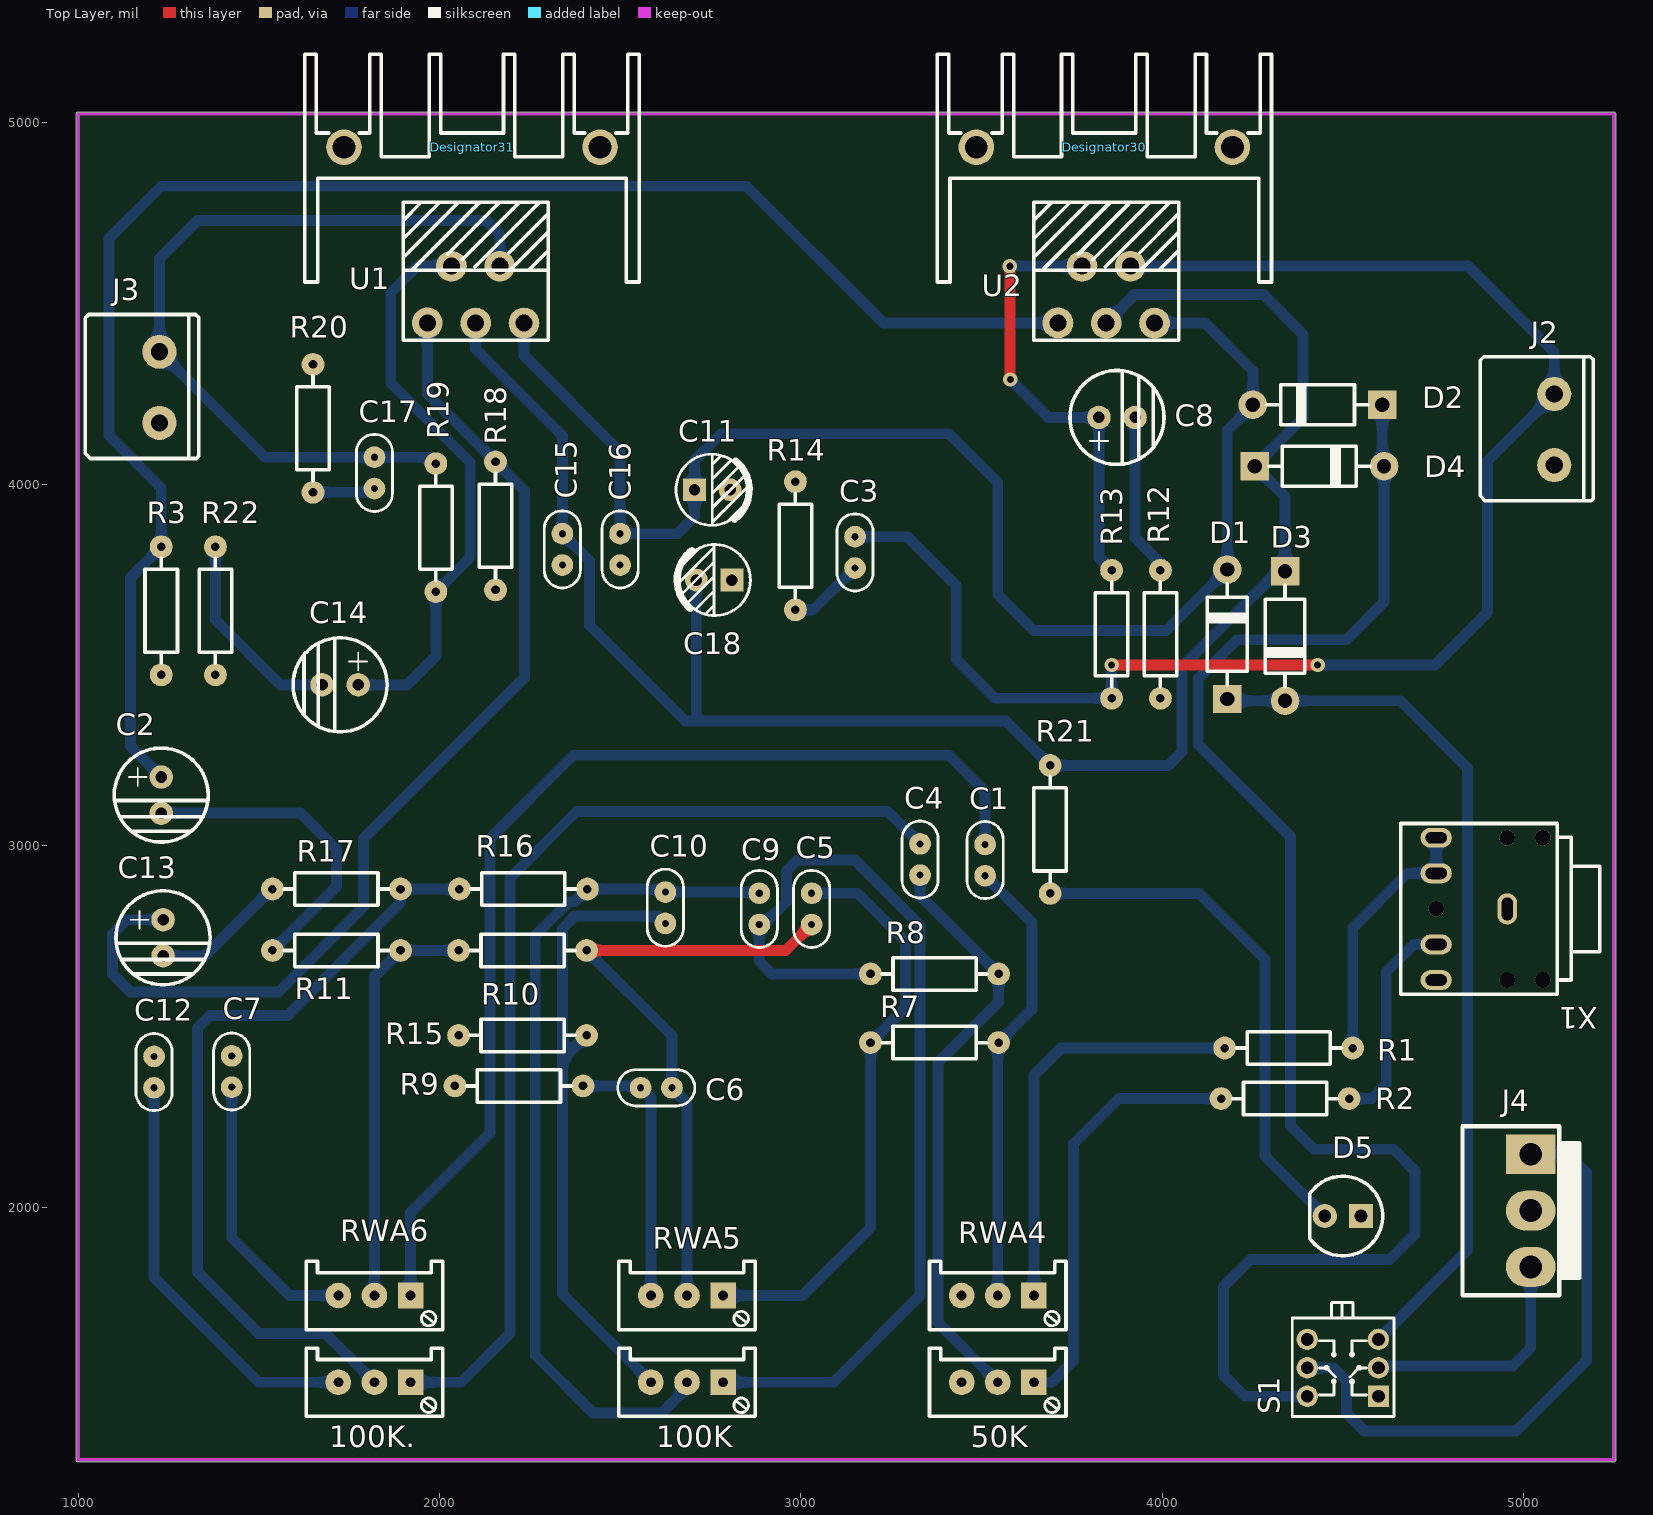
[diagram p0: Top Layer view]
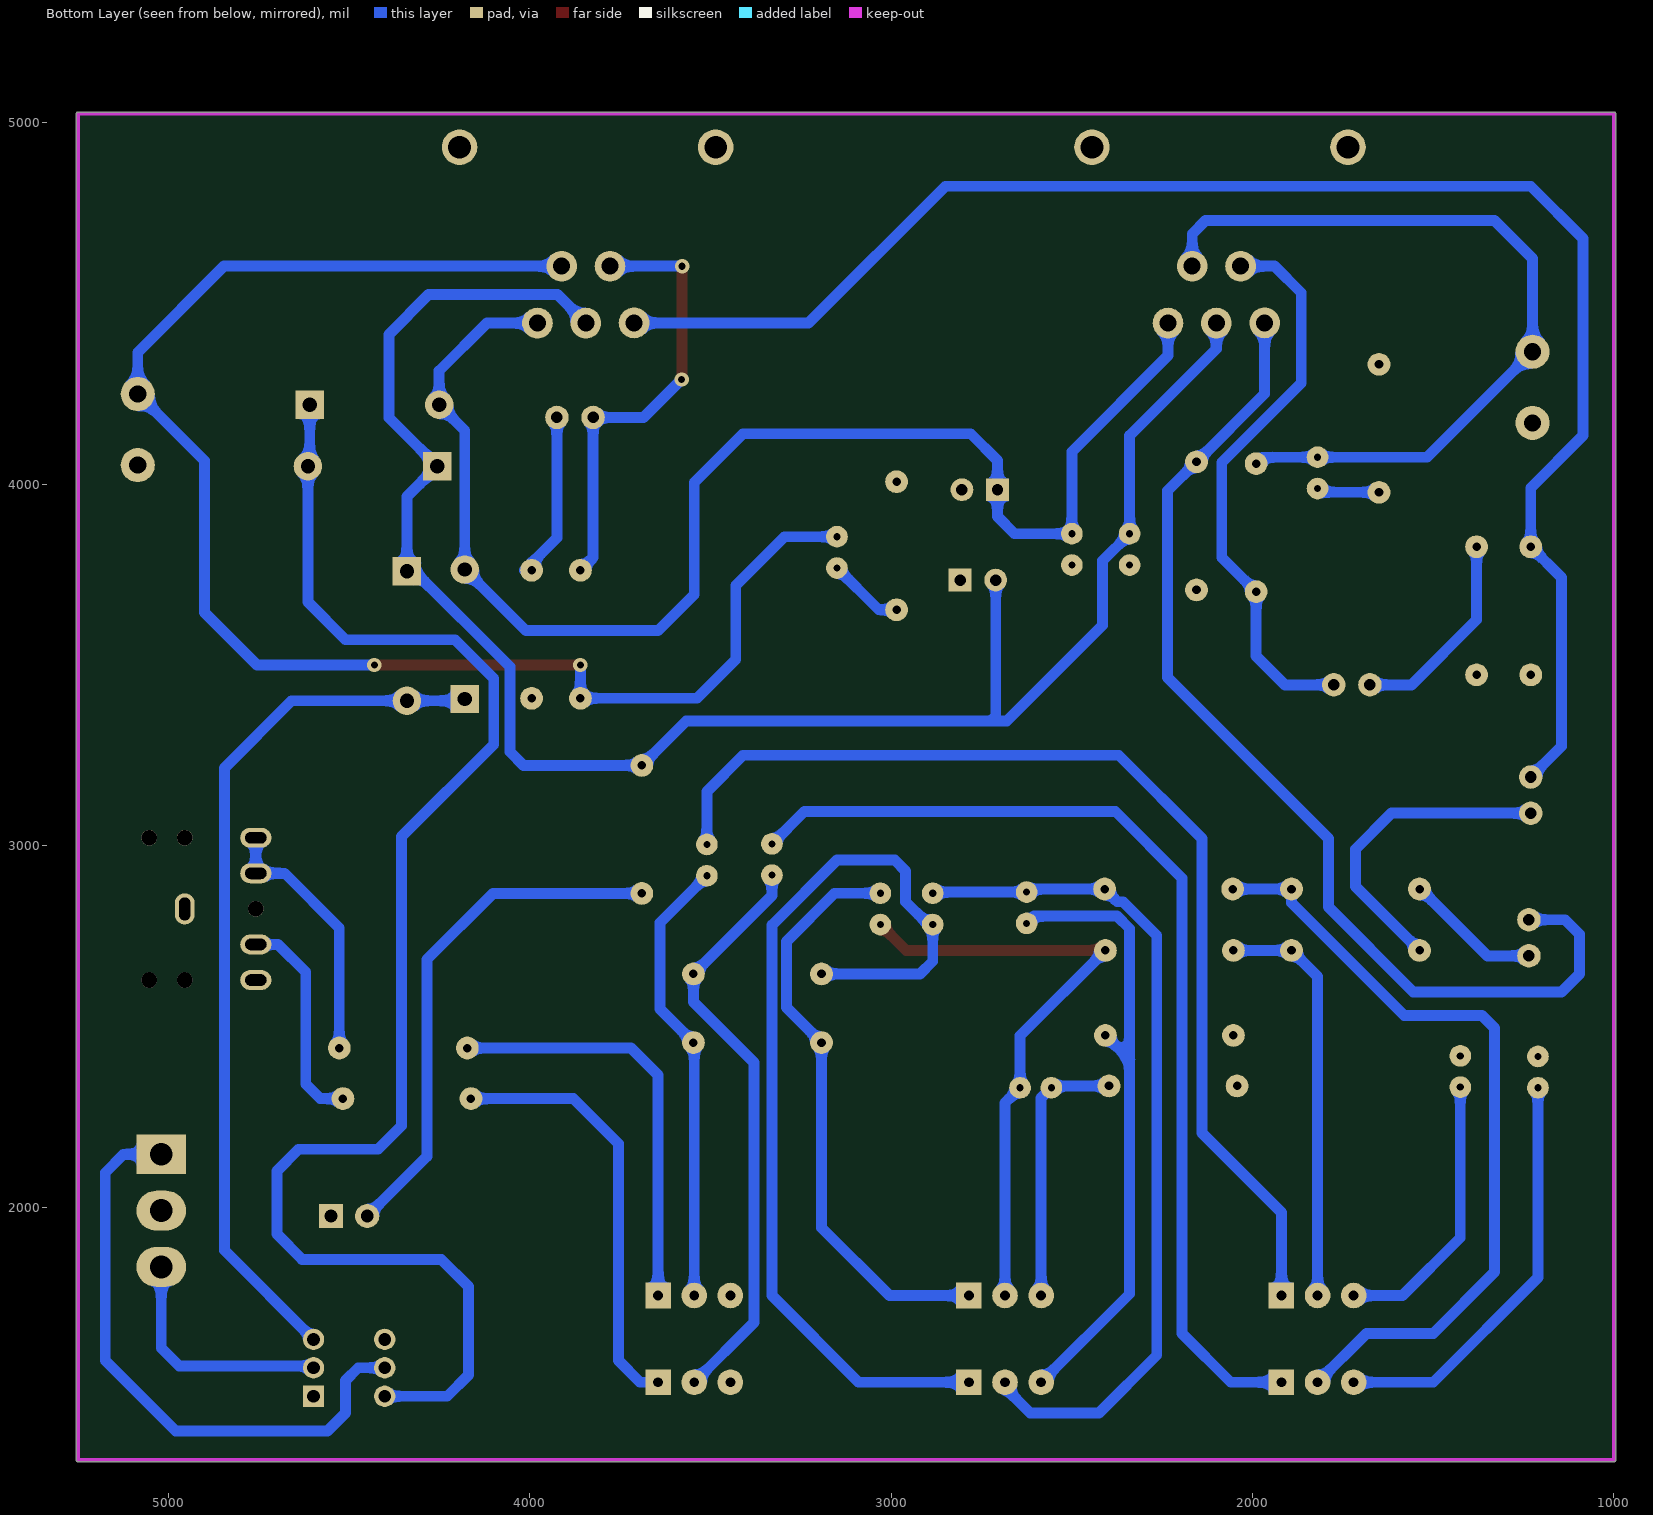
[diagram p1: Bottom Layer view, seen from below]
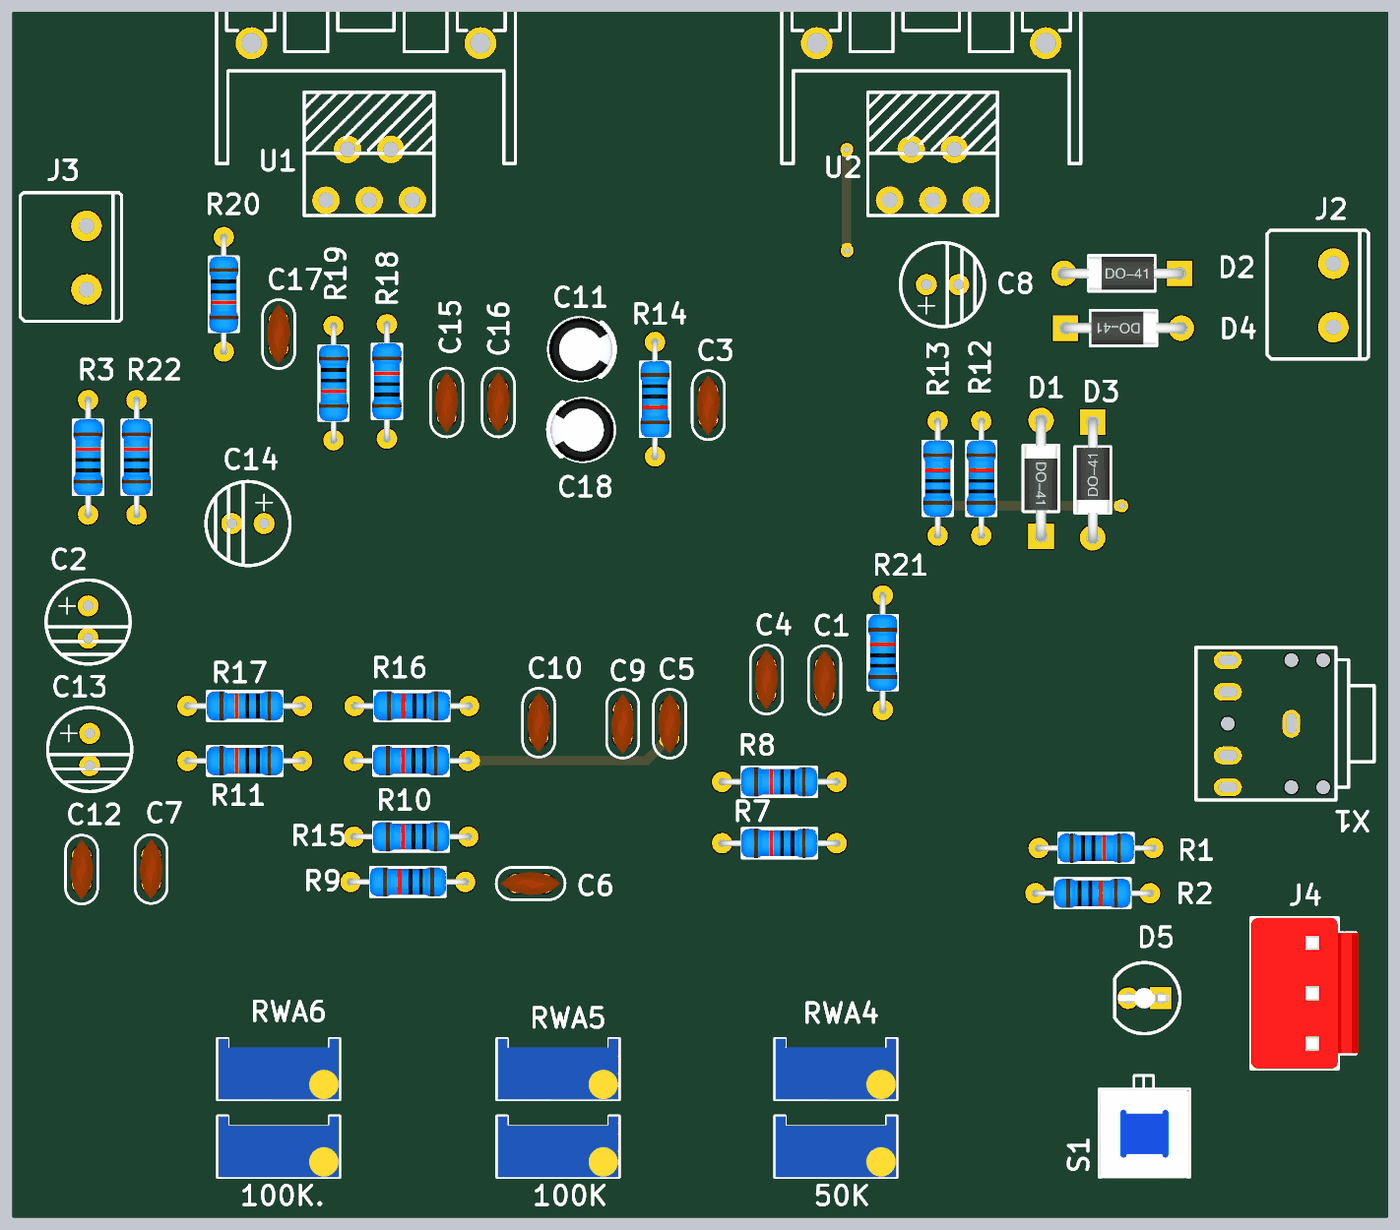
[diagram p2: 3D render of the assembled board from above, using the file's embedded part models]
# Altium PCB MISC82779.PcbDoc
Units mil, origin at the board's own origin, x right, y up, seen from the top; angles counter-clockwise.
Board outline 4260.03 x 3735.03 mil, 2 copper layers (Top Layer, Bottom Layer); 57 components, 38 nets, 139 pads, 4 vias.

## Layer stack, top to bottom (the 12.6 mil dielectric is the usual default, probably not edited)
Top Solder: solder mask 0.4, Solder Resist, Dk 3.5
Top Layer: signal copper 1.4
Dielectric 1: dielectric 12.6, FR-4, Dk 4.8
Bottom Layer: signal copper 1.4
Bottom Solder: solder mask 0.4, Solder Resist, Dk 3.5

## Board outline
1000,1294.98 cw(c1000,1300) 994.99,1300 994.99,5025 cw(c1000,5025) 1000,5030.02 5250,5030.02 cw(c5250,5025) 5255.02,5025 5255.02,1300 cw(c5250,1300) 5250,1294.98

## Design rules (kind name [scope] priority, off if disabled: settings)
Clearance [All] p1: gap=10
HoleSize [All] p1: absolutevalues=TRUE maxlimit=9999 minlimit=1 maxpercent=80.000 minpercent=20.000
MinimumSolderMaskSliver [All] p1: minsoldermaskwidth=9
PolygonConnect [All] p1: connectstyle=Relief reliefconductorwidth=10 reliefentries=4 polygonreliefangle="90 Angle" airgapwidth=10
RoutingVias [All] p1: holewidth=28 width=50 viastyle="Through Hole" minholewidth=28 minwidth=50 maxholewidth=28 maxwidth=50
SilkToSilkClearance [All] p1: silktosilkclearance=0
SilkToSolderMaskClearance [IsPad] p1: minsilkscreentomaskgap=9 clearancetoexposedcopper=TRUE
SolderMaskExpansion [All] p1: expansion=4
Width [All] p1: maxlimit=30 minlimit=10 preferedwidth=10
26 further rules are at their usual default settings.

## Components (designator, comment, footprint, x,y, rotation, side; value= is the part's Value field where it differs from the comment)
50K "10K" 3296W 3545,1515 r180 top
100K "10K" 3296W 2685,1515 r180 top
100K. "10K" 3296W 1820,1515 r180 top
C1 "222" "CC 2.2*5" 3510,2960 r90 top
C2 "10UF" EC100 1230,3090 r0 top
C3 "224" "CC 2.2*5" 3150,3811.69 r90 top
C4 "222" "CC 2.2*5" 3330,2961.69 r90 top
C5 "223" "CC 2.2*5" 3030,2825 r90 top
C6 "224" "CC 2.2*5" 2600,2330 r0 top
C7 "223" "CC 2.2*5" 1425,2375 r270 top
C8 "10UF" EC100 3925,4185 r90 top
C9 "223" "CC 2.2*5" 2885,2825 r270 top
C10 "224" "CC 2.2*5" 2625,2828.31 r90 top
C11 "2200UF" "CAP 2.5*5*11 - BK" 2755,3985 r0 top
C12 "223" "CC 2.2*5" 1210,2373.31 r270 top
C13 "10UF" EC100 1235,2695 r0 top
C14 "10UF" EC100 1675,3445 r270 top
C15 "104" "CC 2.2*5" 2340,3820 r90 top
C16 "104" "CC 2.2*5" 2500,3820 r90 top
C17 "224" "CC 2.2*5" 1820,4031.69 r90 top
C18 "2200UF" "CAP 2.5*5*11 - BK" 2760,3735 r180 top
D1 "1N4007" DO-41 4180,3585 r90 top
D2 "1N4007" DO-41 4430,4220 r180 top
D3 "1N4007" DO-41 4340,3580 r270 top
D4 "1N4007" DO-41 4435,4050 r0 top
D5 "LED" "LED 5MM-W" 4500,1975 r180 top
Designator30 "Comment" TH-2P_L23.5-W16.8 3840,4875 r0 top
Designator31 "Comment" TH-2P_L23.5-W16.8 2090,4875 r0 top
J2 "socket" DZ 5085,4053.15 r90 top
J3 "socket" DZ 1225,4170 r90 top
J4 "AC+/-12V" VH3.96-3A 5020,2145.91 r270 top
R1 "1K" "RS 1/4W" 4350,2440 r0 top
R2 "1K" "RS 1/4W" 4340,2300 r0 top
R3 "22K" "RS 1/4W" 1230,3650 r90 top
R7 "10K" "RS 1/4W" 3370,2455 r180 top
R8 "10K" "RS 1/4W" 3370,2645 r180 top
R9 "1.5K" "RS 1/4W" 2220,2335 r180 top
R10 "5.6K" "RS 1/4W" 2230,2710 r180 top
R11 "2.2K" "RS 1/4W" 1715,2710 r180 top
R12 "330" "RS 1/4W" 3995,3585 r90 top
R13 "47K" "RS 1/4W" 3860,3585 r90 top
R14 "10" "RS 1/4W" 2985,3830 r270 top
R15 "1.5K" "RS 1/4W" 2230,2475 r180 top
R16 "5.6K" "RS 1/4W" 2232.17,2880 r180 top
R17 "2.2K" "RS 1/4W" 1715,2880 r180 top
R18 "22K" "RS 1/4W" 2155,3885 r90 top
R19 "47K" "RS 1/4W" 1990,3880 r270 top
R20 "10" "RS 1/4W" 1650,4155 r270 top
R21 "10K" "RS 1/4W" 3690,3045 r90 top
R22 "330" "RS 1/4W" 1380,3650 r90 top
RWA4 "10K" 3296W 3545,1755 r180 top
RWA5 "10K" 3296W 2685,1755 r180 top
RWA6 "10K" 3296W 1820,1755 r180 top
S1 "KET 7X7" "KFT DIP-7X7" 4500,1555 r90 top
U1 "TDA2030" TDA2030 2100,4590 r0 top
U2 "TDA2030" TDA2030 3845,4590 r0 top
X1 "STEREO" 3F07 4935.31,2825 r180 top

## Footprints (in the part's own frame and the unit in brackets; to place one, negate y for a bottom-side part, rotate by r counter-clockwise, add the part's x,y. Pads: shape width x height; smd on the part's side, far side on the other; paste and mask are expansions set on the pad)
3F07 [mm]
  oval 1.4x2.2 hole 0.8 slot 1.6 at 90 deg paste+0 mask+0.051: 1(-0.5,0)
  oval 2.2x1.4 hole 0.8 slot 1.5 at 0 deg paste+0 mask+0.051: 2(4.5,5) 3(4.5,2.5) 4(4.5,-2.5) 5(4.5,-5)
  round 1.1 hole 1.1 unplated paste+0: ""(-3,5) ""(-3,-5) ""(-0.5,5) ""(-0.5,-5) ""(4.5,0)
  silkscreen extent -7,-6 7,6
3296W [mm] "Precise Multi-Winding Adjustable Resistor"
  rect 1.8x1.8 hole 0.7: 1(-2.54,0)
  round 1.8 hole 0.7: 2(0,0) 3(2.54,0)
  silkscreen extent -4.8,-2.4 4.8,2.4, body extent -4.75,-2.4 4.75,2.4, height 11.52
"CAP 2.5*5*11 - BK" [mm] "脚距2.5mm直径5mm高度11mm"
  rect 1.6x1.6 hole 0.8: 1(-1.25,0)
  round 1.6 hole 0.8: 2(1.25,0)
  silkscreen extent -2.55,-2.5 2.6,2.5, body extent -2.5,-2.5 2.51,2.5, height 11.04
"CC 2.2*5" [mil] "脚距2.2mm直径5mm"
  round 60 hole 19.68: 1(-43.31,0) 2(43.31,0)
  silkscreen extent -107,-50 107,50, body extent -94,-36 94,36, height 189
DO-41 [mm] "2.6*9.1mm(直径，脚距）"
  rect 2x2 hole 1: 1(-4.55,0)
  round 2 hole 1: 2(4.55,0)
  silkscreen extent -3.56,-1.4 3.56,1.4, body extent -4.92,-1.29 4.98,1.31, height 2.65
DZ [mm]
  round 2.4 hole 1.2: 1(0,0) 2(5,0)
  silkscreen extent -2.5,-2.75 7.62,5.21
EC100 [mil]
  round 65 hole 32: 1(0,100) 2(0,0)
  silkscreen extent -130,-80 130,180
"KFT DIP-7X7" [mm] "自锁开关，规格：7*7mm"
  rect 1.5x1.5 hole 0.9: 1(-2,-2.5)
  round 1.5 hole 0.9: 2(0,-2.5) 3(2,-2.5) 4(2,2.5) 5(0,2.5) 6(-2,2.5)
  silkscreen extent -3.42,-3.58 4.58,3.56, body extent -3.5,-3.5 3.5,3.5, height 11.2
"LED 5MM-W" [mm] "白色5mm直插LED"
  rect 1.7x1.7 hole 0.9: 1(-1.27,0)
  round 1.7 hole 0.9: 2(1.27,0)
  silkscreen extent -2.8,-2.8 2.33,2.8, body extent -2.85,-2.85 2.45,2.85, height 8.75
"RS 1/4W" [mm]
  round 1.6 hole 0.6: 1(-4.5,0) 2(4.5,0)
  silkscreen extent -3.68,-1.14 3.68,1.14, body extent -4.72,-1.16 4.73,1.16, height 2.32
TDA2030 [mil]
  round 85 hole 47.24 paste+0 mask+2: 1(-133.54,-143.46) 2(-66.93,13.78) 3(0,-143.7) 4(66.93,13.78) 5(133.86,-143.7)
  silkscreen extent -201,-191 201,191
TH-2P_L23.5-W16.8 [mm]
  round 2.5 hole 1.6 paste+0 mask+0.05: 1(-8.999,1.47) 2(9.001,1.47)
  silkscreen extent -11.75,-8 11.75,8
VH3.96-3A [mm]
  rect 2.8x3.5 hole 1.6: 1(0,0)
  oval 2.8x3.5 hole 1.6: 2(3.96,0) 3(7.92,0)
  silkscreen extent -1.98,-4.8 9.9,3.4, body extent -1.98,-4.8 9.9,3.6, height 14.6

## Part data
50K 100K 100K. RWA4 RWA5 RWA6: library part RP, "single-gang potentiometer"
C1 C3 C4 C5 C6 C7 C9 C10 C12 C15 C16 C17: library part CC, "ceramic disc capacitor"
C2 C8 C13 C14: library part ECAP
C11 C18: library part CE, "through-hole electrolytic capacitor"
D1 D2 D3 D4: "rectifier diode"
J2 J3: library part 插座
J4: library part VH3
R1 R2 R3 R7 R8 R9 R10 R11 R12 R13 R14 R15 R16 R17 R18 R19 R20 R21 R22: library part R-S, "color-band resistor"
S1: "7*7 self-locking switch"
X1: library part 3F07

## Via types
v1: diameter 40, hole 20, Top Layer to Bottom Layer, 4 vias

## Nets (pads, with @x,y where several pads share a name; then routed paths per layer and width w, separated by ;. In a path a pad name is that pad's centre, name@x,y a point inside that pad or via, vN(x,y) a via of type N, cw(c..) or ccw(c..) an arc to the next point about the centre after c; other vN are vias at no path point)
+17V: C11.1 C16.2 D1.2 D2.2 U1.5 U2.5 | length 3962.1
  Bottom Layer w30: U1.5 2233.86,4356.14 2500,4090 C16.2 2658.31,3863.31 2705.79,3910.79 C11.1 2705.79,4065.79 2780,4140 3410,4140 3545,4005 3545,3695 3645,3595 4010.87,3595 D1.2 4180,4149.13 D2.2 4250.87,4314.13 4118.7,4446.3 U2.5
-17V: C15.2 C18.2 D3.1 D4.1 R21.2 U1.3 U2.3 | length 5177.8
  Bottom Layer w30: U1.3 2100,4375 2340,4135 C15.2 2415,3788.31 2415,3610 2680,3345 2725,3345 ; C18.2 2710.79,3359.21 2725,3345 ; U2.3 3923.7,4525 4280,4525 4390,4415 4390,4184.13 D4.1 4340,3965.87 D3.1 4319.13,3759.13 4055,3495 4055,3260 4017.17,3222.17 R21.2 3567.17,3345 2725,3345
GND: 50K.3 C7.1 C11.2 C12.1 C15.1 C16.1 C18.1 D5.1 J2.1 J3.1 J4.2 R3.1 R9.2 R12.1 R14.1 R15.2 R18.1 R20.1 R22.1 RWA4.3 X1.1
Net50K_1: 50K.1 R2.1 | length 1194.5
  Bottom Layer w30: 50K.1 3695,1515 3755,1575 3755,2175 3880,2300 R2.1
Net50K_2: 50K.2 C4.1 R8.1 | length 1630.9
  Bottom Layer w30: C4.1 3330,2862.17 R8.1 3547.17,2567.17 3380,2400 3380,1680 50K.2
Net100K._1: 100K..1 C4.2 | length 2839.8
  Bottom Layer w30: 100K..1 2060,1515 2195,1650 2195,2910 2380,3095 3240,3095 C4.2
Net100K._2: 100K..2 R16.2 R17.1 | length 2198
  Bottom Layer w30: 100K..2 1685,1650 1500,1650 1330,1820 1330,2495 1365,2530 1580,2530 1892.17,2842.17 R17.1 R16.2
Net100K._3: 100K..3 C12.2 | length 1155.1
  Bottom Layer w30: C12.2 1210,1805 1500,1515 100K..3
Net100K_1: 100K.1 C9.2 R8.2 | length 2741.5
  Bottom Layer w30: 100K.1 3090,1515 3330,1755 3330,2780 3150,2960 2990,2960 2960,2930 2960,2845 2905,2790 2885,2790 C9.2 2885,2680 2920,2645 R8.2
Net100K_2: 100K.2 C9.1 C10.2 R16.1 | length 2369.9
  Bottom Layer w30: 100K.2 2685,1500 2615,1430 2425,1430 2265,1590 2265,2751.57 2358.43,2845 2374.33,2845 R16.1 2616.61,2880 C10.2 2881.69,2871.61 C9.1
Net100K_3: 100K.3 C10.1 R15.1 | length 1759.3
  Bottom Layer w30: R15.1 2340,2407.83 ; 100K.3 2340,1760 2340,2407.83 ; C10.1 2605,2805 2375,2805 2340,2770 2340,2407.83
NetC1_1: C1.1 R7.1 RWA4.2 | length 1254.9
  Bottom Layer w30: C1.1 3640,2786.69 3640,2547.83 R7.1 3545,2452.83 RWA4.2
NetC1_2: C1.2 RWA6.1 | length 3009.5
  Bottom Layer w30: RWA6.1 1920,1985 2140,2205 2140,3020 2370,3250 3410,3250 3510,3150 C1.2
NetC2_1: C2.1 R3.2 U2.1 | length 4463.8
  Bottom Layer w30: C2.1 1145,3275 1145,3742.17 R3.2 1230,3990 1085,4135 1085,4680 1230,4825 2850,4825 3228.46,4446.54 U2.1
NetC2_2: C2.2 R11.2 | length 879.8
  Bottom Layer w30: C2.2 1615,3090 1715,2990 1715,2887.17 R11.2
NetC3_1: C3.1 R14.2 | length 212.9
  Bottom Layer w30: R14.2 3034.45,3652.83 C3.1
NetC3_2: C3.2 J2.2 R13.1 U2.4 | length 4276.1
  Top Layer w30: v1(3860,3500) v1(4430,3500)
  Bottom Layer w30: C3.2 3295,3855 3430,3720 3430,3515 3537.17,3407.83 R13.1 v1(3860,3500) ; U2.4 4846.22,4603.78 5085,4365 J2.2 4900,4065 4900,3645 4755,3500 v1(4430,3500)
NetC5_1: C5.1 C6.2 R10.1 RWA5.2 | length 1722.6
  Top Layer w30: R10.1 2958.31,2710 C5.1
  Bottom Layer w30: R10.1 2643.31,2473.86 C6.2 2685,2288.31 RWA5.2
NetC5_2: C5.2 R7.2 RWA5.1 | length 1633.3
  Bottom Layer w30: RWA5.1 3005,1755 3192.83,1942.83 R7.2 3290,2552.17 3290,2735 3156.69,2868.31 C5.2
NetC6_1: C6.1 R9.1 RWA5.3 | length 748.3
  Bottom Layer w30: R9.1 2551.69,2335 C6.1 2585,2301.69 RWA5.3
NetC7_2: C7.2 RWA6.3 | length 778
  Bottom Layer w30: C7.2 1425,1915 1585,1755 RWA6.3
NetC8_1: C8.1 R13.2 U2.2 | length 1239.4
  Top Layer w30: v1(3578.78,4603.78) 3578.78,4291.22 v1(3580,4290)
  Bottom Layer w30: v1(3578.78,4603.78) U2.2 ; v1(3580,4290) 3685,4185 C8.1 3825,3797.17 R13.2
NetC8_2: C8.2 R12.2 | length 460.1
  Bottom Layer w30: C8.2 3925,3852.17 R12.2@4015,3762.17
NetC13_1: C13.1 R18.2 U1.1 | length 2991.7
  Bottom Layer w30: C13.1 1135,2795 1095,2755 1095,2645 1145,2595 1555,2595 1790,2830 1790,3020 2235,3465 2235,3982.17 R18.2 1966.46,4250.71 U1.1
NetC13_2: C13.2 R17.2 | length 379.5
  Bottom Layer w30: C13.2 1350,2695 1535,2880 R17.2
NetC14_1: C14.1 R19.2 U1.2 | length 1582.2
  Bottom Layer w30: C14.1 1910,3445 1990,3525 R19.2 2085,3797.83 2085,4060 1865,4280 1865,4530 1938.78,4603.78 U1.2
NetC14_2: C14.2 R22.2 | length 571.7
  Bottom Layer w30: R22.2 1380,3625 1560,3445 C14.2
NetC17_1: C17.1 R20.2 | length 174.4
  Bottom Layer w30: R20.2 1809.45,3977.83 C17.1
NetC17_2: C17.2 J3.2 R19.1 U1.4 | length 2241.4
  Bottom Layer w30: R19.1 1972.17,4075 C17.2 1516.85,4075 J3.2 1225,4625 1330,4730 2130,4730 2166.93,4693.07 U1.4
NetD1_1: D1.1 D3.2 S1.3 | length 2427.5
  Bottom Layer w30: D1.1 4185,3400.87 D3.2 4659.13,3400.87 4845,3215 4845,1880.32 S1.3
NetD2_1: D2.1 D4.2 S1.6 | length 4155.6
  Bottom Layer w30: S1.6 4228.74,1476.26 4170,1535 4170,1780 4245,1855 4630,1855 4700,1925 4700,2100 4640,2160 4420,2160 4355,2225 4355,3025 4100,3280 4100,3462.57 4207.43,3570 4510,3570 4614.13,3674.13 D4.2 4609.13,4055 D2.1
NetD5_2: D5.2 R21.1 | length 1449.1
  Bottom Layer w30: R21.1 4102.17,2867.83 4285,2685 4285,2140 D5.2
NetJ4_1: J4.1 S1.5 | length 1675.5
  Bottom Layer w30: S1.5 4475,1555 4510,1520 4510,1430 4560,1380 4980,1380 5175,1575 5175,2095 5124.09,2145.91 J4.1
NetJ4_3: J4.3 S1.2 | length 661.4
  Bottom Layer w30: S1.2@4603.43,1560 4970,1560 5020,1610 J4.3
NetR1_1: R1.1 RWA4.1 | length 1168.9
  Bottom Layer w30: RWA4.1 3645,2365 3720,2440 R1.1
NetR1_2: R1.2 X1.4 X1.5 | length 724.2
  Bottom Layer w30: R1.2 4527.17,2772.17 4678.43,2923.43 X1.4 X1.5
NetR2_2: R2.2 X1.3 | length 599.3
  Bottom Layer w30: R2.2 4580,2300 4620,2340 4620,2650 4696.57,2726.57 X1.3
NetR10_2: R10.2 R11.1 RWA6.2 | length 1145.6
  Bottom Layer w30: RWA6.2 1820,2637.83 R11.1 R10.2
pads on no net: Designator30.1 Designator30.2 Designator31.1 Designator31.2 S1.1 S1.4 X1. X1.2

## Keep-outs
Keep-Out Layer:
  lines w10: 1000,4980 1000,5025 5250,5025 5250,1300 5200,1300 1000,1300 1000,4995